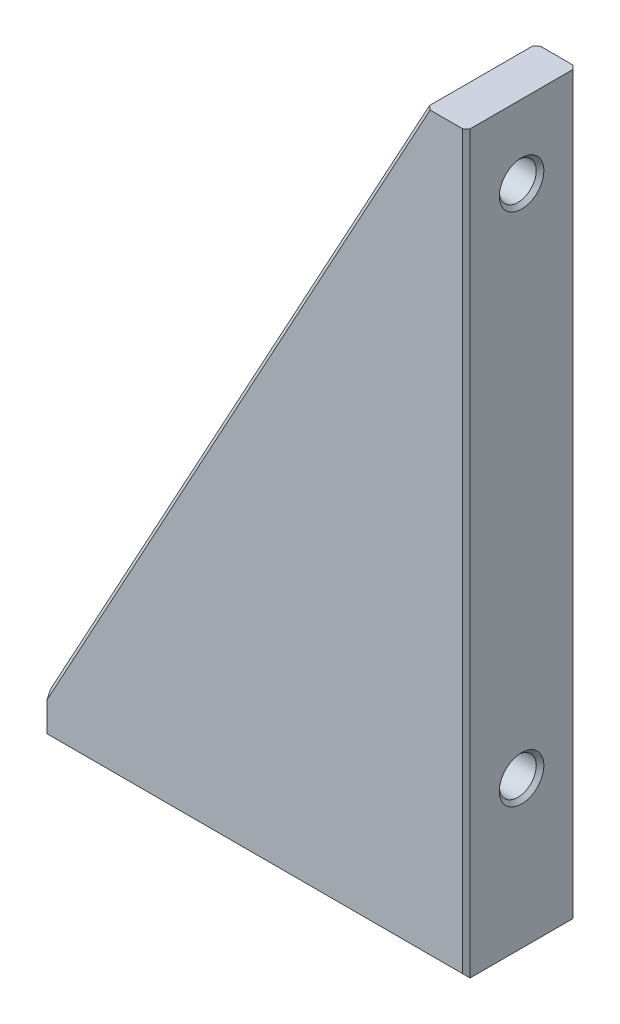
from build123d import *

# Parameters (mm, degrees)
EXTRUDE_1_DEPTH              = 15
HOLE_WIZARD_M6_1_D           = 5
HOLE_WIZARD_M6_1_DEPTH       = 15
HOLE_WIZARD_M6_1_CSINK_D     = 6.5
HOLE_WIZARD_M6_1_CSINK_ANGLE = 92
HOLE_WIZARD_M6_1_TIP         = 1.502151548
HOLE_WIZARD_M6_2_D           = 5
HOLE_WIZARD_M6_2_DEPTH       = 15
HOLE_WIZARD_M6_2_CSINK_D     = 6.05
HOLE_WIZARD_M6_2_CSINK_ANGLE = 92
HOLE_WIZARD_M6_2_TIP         = 1.502151548
CHAMFER_1_SIZE               = 0.5
SKETCH_7_W                   = 5.5
SKETCH_7_H                   = 10.083333333
SKETCH_7_W_2                 = 3
SKETCH_7_H_2                 = 20
CUT_EXTRUDE_1_DEPTH          = 127.194294641


with BuildPart() as part:
    # 草图1 → 凸台-拉伸1 (new body)
    with BuildSketch(Plane.XY):
        Polygon((0, 0), (60, 0), (60, 110), align=None)
    extrude(amount=EXTRUDE_1_DEPTH)

    # M6 螺纹孔1
    with Locations(Plane(origin=(0, 0, 0), x_dir=(-1, 0, 0), z_dir=(0, -1, 0))):
        with Locations((-48, -7.5), (-12, -7.5)):
            CounterSinkHole(HOLE_WIZARD_M6_1_D / 2, HOLE_WIZARD_M6_1_CSINK_D / 2, depth=HOLE_WIZARD_M6_1_DEPTH, counter_sink_angle=HOLE_WIZARD_M6_1_CSINK_ANGLE)
            with Locations((0, 0, -(HOLE_WIZARD_M6_1_DEPTH + HOLE_WIZARD_M6_1_TIP / 2))):  # 118° drill point
                Cone(0, HOLE_WIZARD_M6_1_D / 2, HOLE_WIZARD_M6_1_TIP, mode=Mode.SUBTRACT)

    # M6 螺纹孔2
    with Locations(Plane(origin=(60, 0, 0), x_dir=(0, 0, -1), z_dir=(1, 0, 0))):
        with Locations((-7.5, 20), (-7.5, 90)):
            CounterSinkHole(HOLE_WIZARD_M6_2_D / 2, HOLE_WIZARD_M6_2_CSINK_D / 2, depth=HOLE_WIZARD_M6_2_DEPTH, counter_sink_angle=HOLE_WIZARD_M6_2_CSINK_ANGLE)
            with Locations((0, 0, -(HOLE_WIZARD_M6_2_DEPTH + HOLE_WIZARD_M6_2_TIP / 2))):  # 118° drill point
                Cone(0, HOLE_WIZARD_M6_2_D / 2, HOLE_WIZARD_M6_2_TIP, mode=Mode.SUBTRACT)

    # 倒角1
    chamfer_1_edges = [part.edges().sort_by_distance(p)[0] for p in [
        (60, 55, 15),
        (60, 55, 0),
        (30, 55, 15),
        (30, 0, 0),
        (30, 55, 0),
        (30, 0, 15),
    ]]
    chamfer(chamfer_1_edges, length=CHAMFER_1_SIZE)

    # 草图7 → 切除-拉伸1 (cut, through all)
    with BuildSketch(Plane.XY.offset(15)):
        with Locations((57.25, 104.958333334)):
            Rectangle(SKETCH_7_W, SKETCH_7_H)
        with Locations((1.5, 10)):
            Rectangle(SKETCH_7_W_2, SKETCH_7_H_2)
    extrude(amount=-CUT_EXTRUDE_1_DEPTH, mode=Mode.SUBTRACT)


solid = part.part
